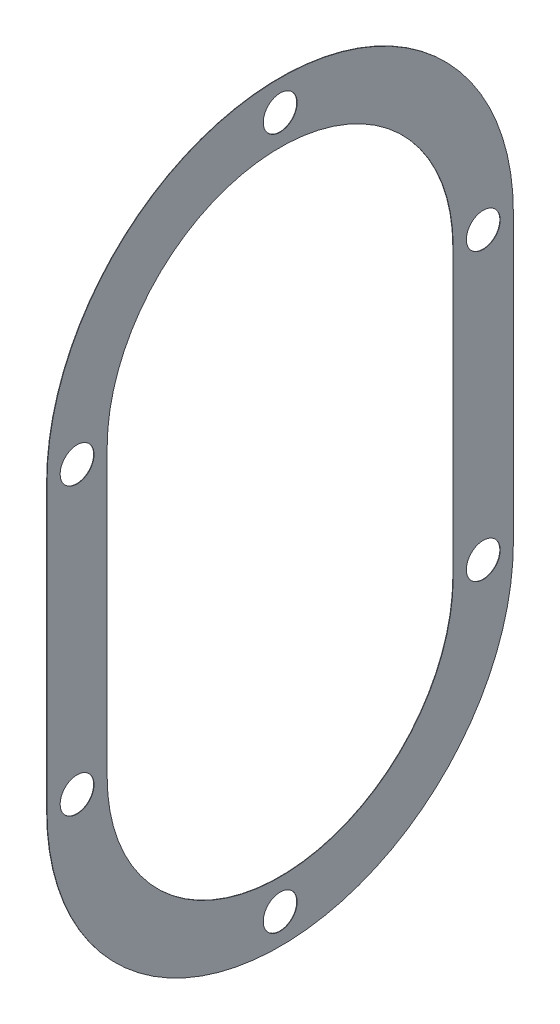
SolidWorks part; units mm, degrees
ref_plane "Front Plane" through (0, 0, 0) normal (0, 0, 1) x (1, 0, 0)
ref_plane "Top Plane" through (0, 0, 0) normal (0, 1, 0) x (1, 0, 0)
ref_plane "Right Plane" through (0, 0, 0) normal (1, 0, 0) x (0, 0, -1)
other "Configuration Table"
ref_plane "Plane1" through (0.05, 0, 0) normal (1, 0, 0) x (0, 0, -1)
sketch "Sketch1" plane through (0.05, 0, 0) normal (1, 0, 0) x (0, 0, -1)
  line L0 (23, 19) -> (23, -19)
  line L1 (-23, -19) -> (-23, 19)
  line L2 (31, -19) -> (31, 19)
  line L3 (-31, 19) -> (-31, -19)
  circle A0 centre (27, -19) radius 2.25
  circle A1 centre (27, 19) radius 2.25
  arc A2 (23, -19) -> (-23, -19) centre (0, -19) cw
  arc A3 (-23, 19) -> (23, 19) centre (0, 19) cw
  arc A4 (-31, -19) -> (31, -19) centre (0, -19) ccw
  arc A5 (31, 19) -> (-31, 19) centre (0, 19) ccw
  circle A6 centre (0, 46) radius 2.25
  circle A7 centre (-27, 19) radius 2.25
  circle A8 centre (-27, -19) radius 2.25
  circle A9 centre (0, -46) radius 2.25
extrude "Boss-Extrude1" add sketch "Sketch1" against normal blind 0.05
